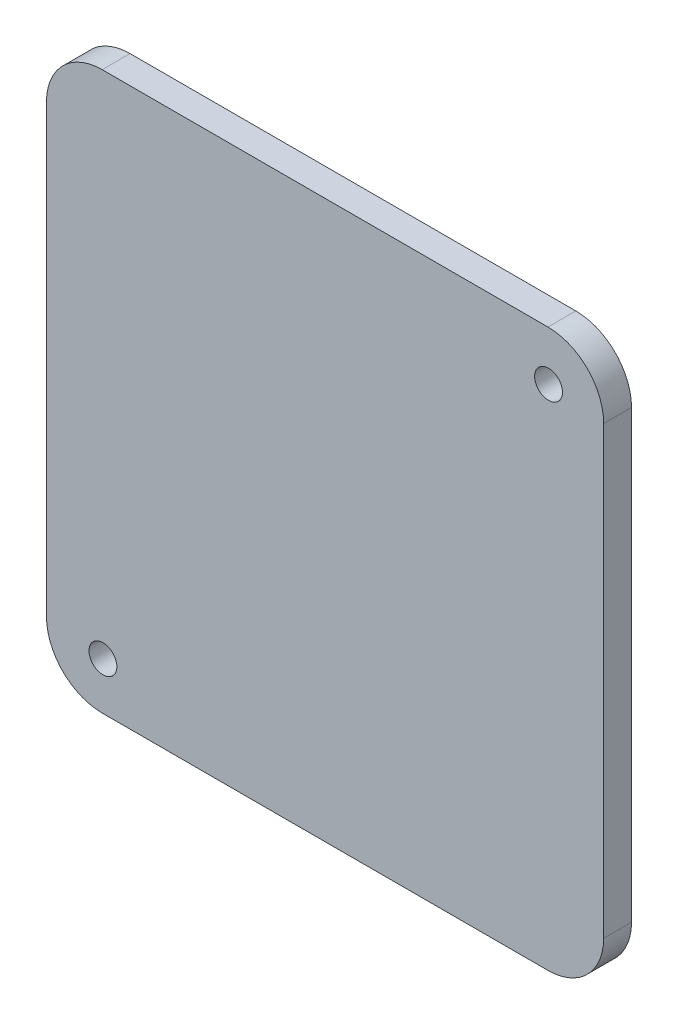
SolidWorks part; units mm, degrees
ref_plane "Front Plane" through (0, 0, 0) normal (0, 0, 1) x (1, 0, 0)
ref_plane "Top Plane" through (0, 0, 0) normal (0, 1, 0) x (1, 0, 0)
ref_plane "Right Plane" through (0, 0, 0) normal (1, 0, 0) x (0, 0, -1)
sketch "Sketch1" plane through (0, 0, 0) normal (0, 0, 1) x (1, 0, 0)
  line L1 (-10, 10) -> (10, 10)
  line L2 (-10, 10) -> (-10, -10)
  line L3 (-10, -10) -> (10, -10)
  line L4 (10, 10) -> (10, -10)
  line L5 (0, -10) -> (0, 10) construction
  line L6 (-10, 0) -> (10, 0) construction
  point P0 (0, 0)
  dimension "D1" = 20
  dimension "D2" = 20
extrude "Boss-Extrude1" add sketch "Sketch1" along normal blind 1
sketch "Sketch2" plane through (0, 0, 1) normal (0, 0, 1) x (1, 0, 0)
  circle A0 centre (-7.9733, -8.2974) radius 0.5
  circle A1 centre (8.0214, 8.2304) radius 0.5
  dimension "D2" = 1
  dimension "D3" = 1
  dimension "D1" = 23
extrude "Cut-Extrude1" cut sketch "Sketch2" against normal through all
fillet "Fillet1" radius 2 4 edges at (10, -10, 0.5) (-10, 10, 0.5) (10, 10, 0.5) (-10, -10, 0.5)
